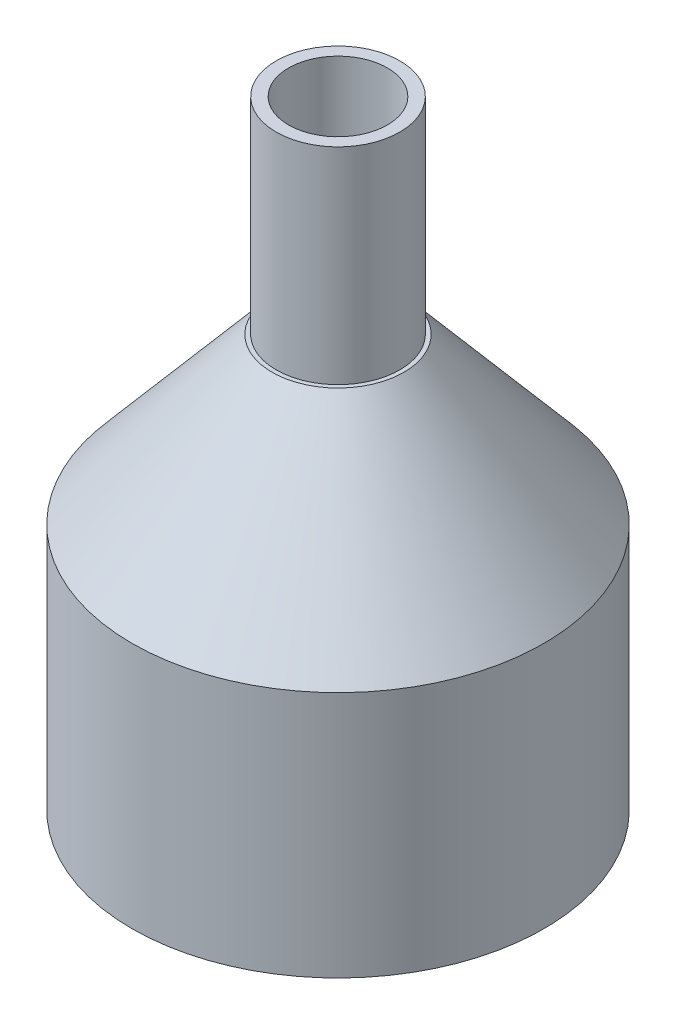
SolidWorks part; units mm, degrees
ref_plane "Front Plane" through (0, 0, 0) normal (0, 0, 1) x (1, 0, 0)
ref_plane "Top Plane" through (0, 0, 0) normal (0, 1, 0) x (1, 0, 0)
ref_plane "Right Plane" through (0, 0, 0) normal (1, 0, 0) x (0, 0, -1)
sketch "Sketch1" plane through (0, 0, 0) normal (0, 1, 0) x (1, 0, 0)
  circle A0 centre (0, 0) radius 25
  dimension "D1" = 50
extrude "Boss-Extrude1" add sketch "Sketch1" along normal blind 50
sketch "Sketch2" plane through (0, 50, 0) normal (0, 1, 0) x (1, 0, 0)
  circle A0 centre (0, 0) radius 7.5
  dimension "D1" = 15
extrude "Boss-Extrude2" add sketch "Sketch2" along normal blind 25
chamfer "Chamfer1" distance 20 distance2 17 1 edges at (0, 50, 25)
sketch "Sketch3" plane through (0, 75, 0) normal (0, 1, 0) x (1, 0, 0)
  circle A0 centre (0, 0) radius 6
  dimension "D1" = 12
extrude "Cut-Extrude1" cut sketch "Sketch3" against normal through all
sketch "Sketch4" plane through (0, 0, 0) normal (0, -1, 0) x (1, 0, 0)
  circle A0 centre (0, 0) radius 21.4533
extrude "Cut-Extrude2" cut sketch "Sketch4" against normal blind 15
